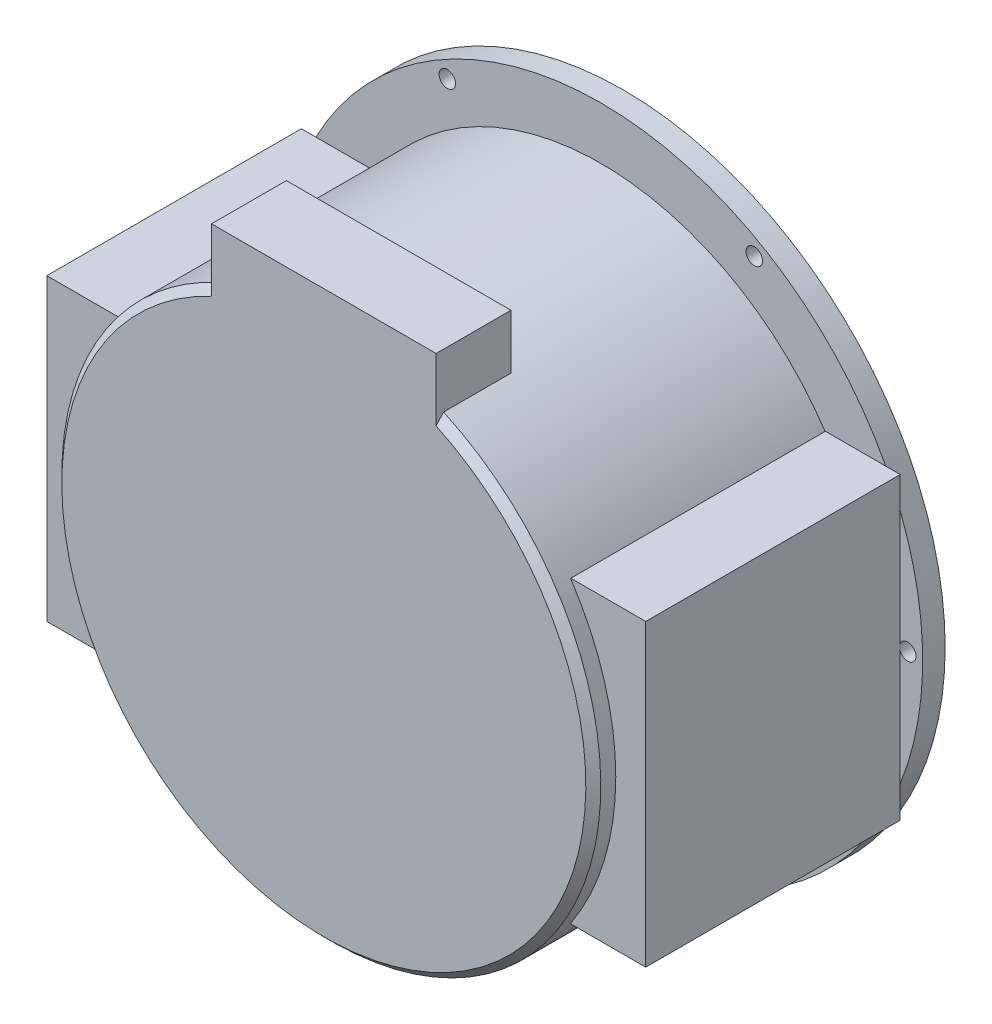
SolidWorks part; units mm, degrees
ref_plane "Front Plane" through (0, 0, 0) normal (0, 0, 1) x (1, 0, 0)
ref_plane "Top Plane" through (0, 0, 0) normal (0, 1, 0) x (1, 0, 0)
ref_plane "Right Plane" through (0, 0, 0) normal (1, 0, 0) x (0, 0, -1)
sketch "Sketch1" plane through (0, 0, 0) normal (0, 0, 1) x (1, 0, 0)
  circle A0 centre (0, 0) radius 180
  dimension "D1" = 360
extrude "Boss-Extrude1" add sketch "Sketch1" along normal mid plane 200
sketch "Sketch2" plane through (0, 0, -100) normal (0, 0, -1) x (-1, 0, 0)
  circle A0 centre (0, 0) radius 25
  dimension "D1" = 50
extrude "Cut-Extrude1" cut sketch "Sketch2" against normal blind 80
sketch "Sketch3" plane through (0, 0, 100) normal (0, 0, 1) x (1, 0, 0)
  line L1 (-75, 200) -> (75, 200)
  line L2 (-75, 200) -> (-75, 137.581)
  line L3 (-75, 137.581) -> (75, 137.581)
  line L4 (75, 200) -> (75, 137.581)
  dimension "D1" = 150
  dimension "D2" = 75
  dimension "D3" = 200
extrude "Boss-Extrude3" add sketch "Sketch3" against normal blind 50
sketch "Sketch4" plane through (0, 0, -100) normal (0, 0, -1) x (-1, 0, 0)
  line L0 (-102.5, 177.5352) -> (0, 0) construction
  line L1 (0, 0) -> (0, 89.5531) construction
  circle A0 centre (0, 0) radius 215
  circle A1 centre (0, 0) radius 180
  circle A2 centre (0, 0) radius 180
  circle A3 centre (-102.5, 177.5352) radius 5.5
  circle A4 centre (102.5, 177.5352) radius 5.5
  circle A5 centre (205, 0) radius 5.5
  circle A6 centre (102.5, -177.5352) radius 5.5
  circle A7 centre (-102.5, -177.5352) radius 5.5
  circle A8 centre (-205, 0) radius 5.5
  point P19 (0, 0)
  dimension "D2" = 430
  dimension "D3" = 11
  dimension "D4" = 205
  dimension "D5" = 30
  dimension "D1" = 0
  dimension "D6" = 6
extrude "Boss-Extrude4" add sketch "Sketch4" against normal blind 15
chamfer "Chamfer1" distance 5 angle 45 1 edges at (0, -180, 100)
sketch "Sketch5" plane through (0, 0, 0) normal (1, 0, 0) x (0, 0, -1)
  line L0 (85, 215) -> (85, -215) construction
  line L1 (-85, 100) -> (85, 100)
  line L2 (-85, 100) -> (-85, -100)
  line L3 (-85, -100) -> (85, -100)
  line L4 (85, 100) -> (85, -100)
  line L5 (-85, 100) -> (85, -100) construction
  line L6 (-85, -100) -> (85, 100) construction
  point P0 (0, 0)
  dimension "D1" = 200
extrude "Boss-Extrude5" add sketch "Sketch5" along normal blind 50 from offset 150
mirror "Mirror1" about plane through (0, 0, 0) normal (1, 0, 0) of "Boss-Extrude5"
